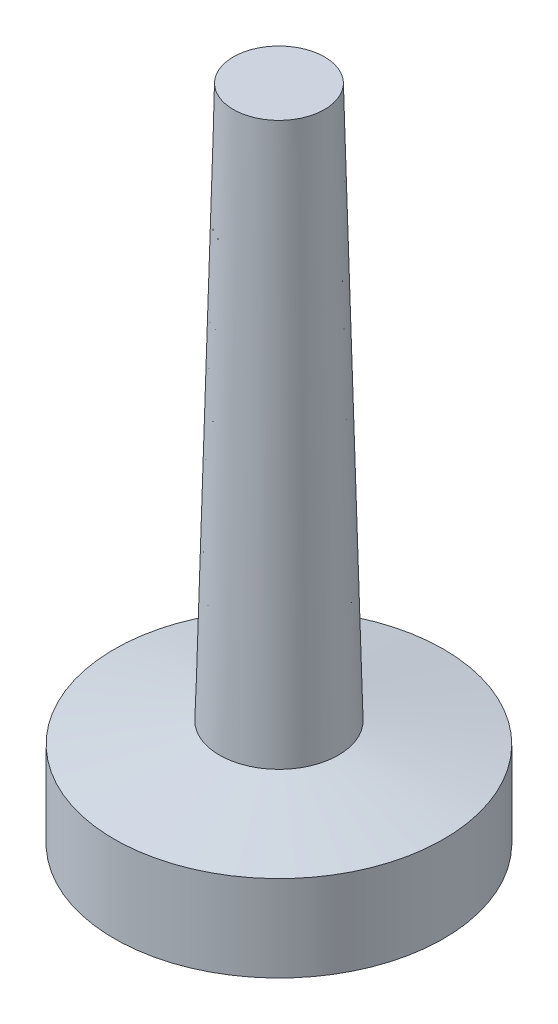
from build123d import *

# Parameters (mm, degrees)
SKETCH_2_R          = 17.5
CUT_EXTRUDE_1_DEPTH = 10
SKETCH_3_R          = 7.5
CUT_EXTRUDE_2_DEPTH = 10


with BuildPart() as part:
    # 草图1 → 旋转1 (revolve)
    with BuildSketch(Plane(origin=(0, 0, 0), x_dir=(0, 0, -1), z_dir=(1, 0, 0))):
        Polygon((0, 0), (0, 130), (9, 130), (11.75, 21), (32.5, 17), (32.5, 0), align=None)
    revolve(axis=Axis((0, 0, 0), (0, 1, 0)))

    # 草图2 → 切除-拉伸1 (cut)
    with BuildSketch(Plane.XZ):
        with Locations(Location((0, 0, 0), (0, 0, 270))):
            Circle(SKETCH_2_R)
    extrude(amount=-CUT_EXTRUDE_1_DEPTH, mode=Mode.SUBTRACT)

    # 草图3 → 切除-拉伸2 (cut)
    with BuildSketch(Plane.XZ.offset(-10)):
        with Locations(Location((0, 0, 0), (0, 0, 270))):
            Circle(SKETCH_3_R)
    extrude(amount=-CUT_EXTRUDE_2_DEPTH, mode=Mode.SUBTRACT)


solid = part.part
